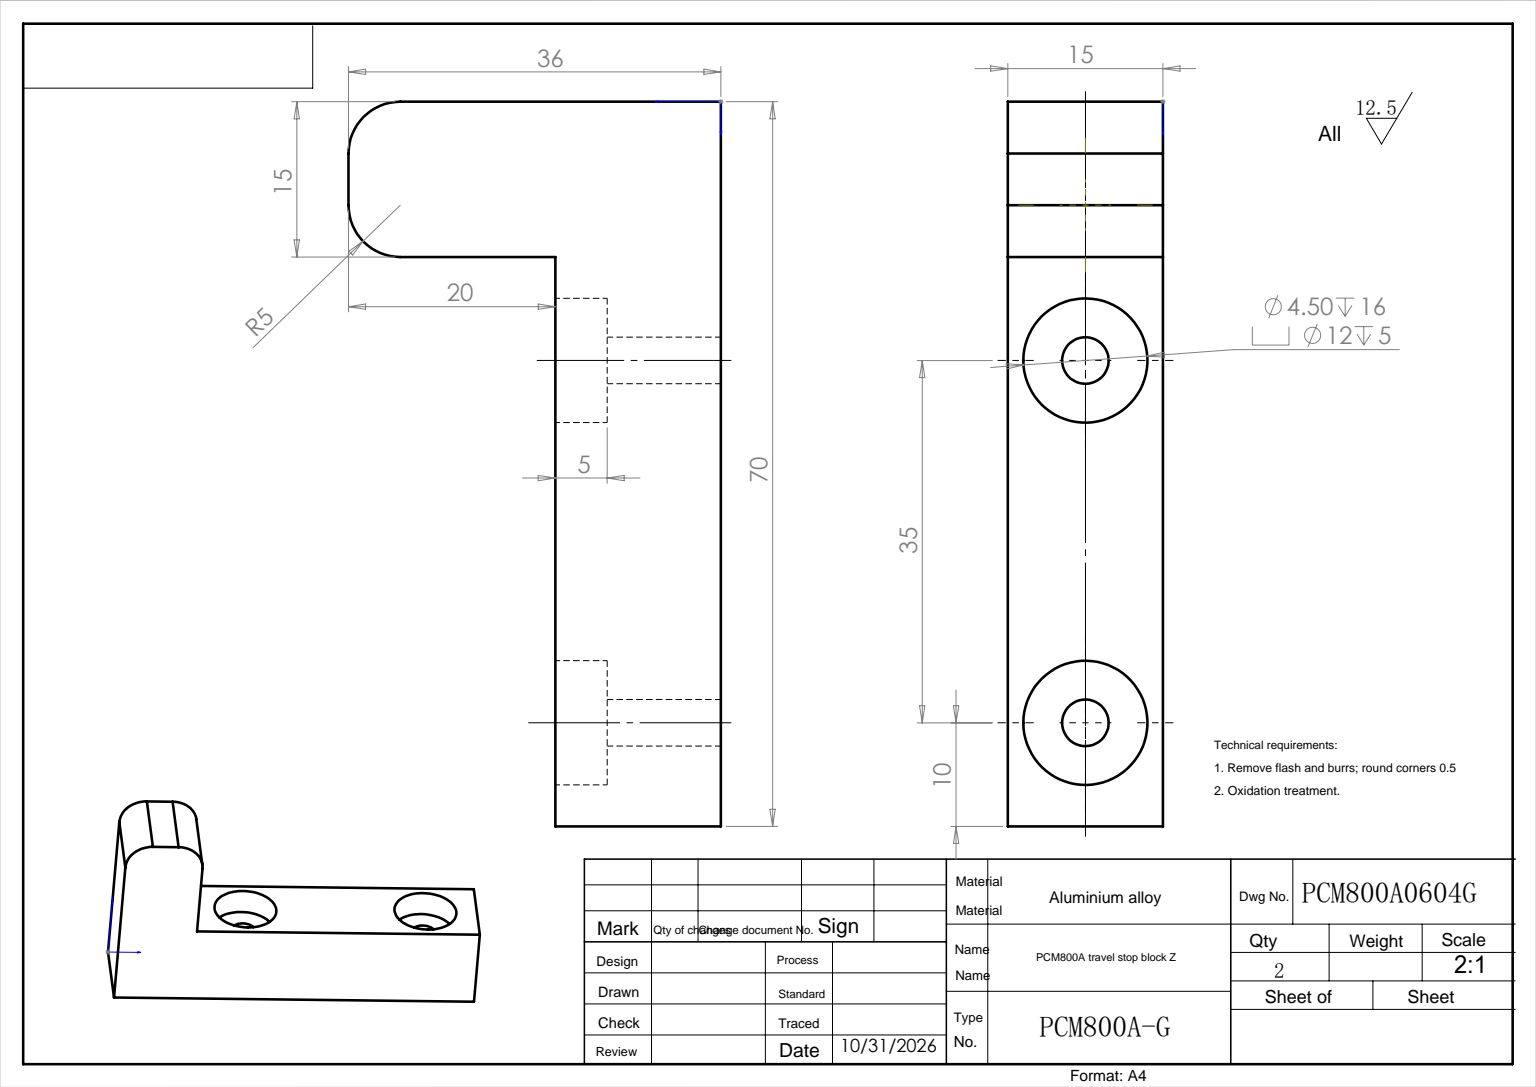
SolidWorks part; units mm, degrees
ref_plane "前视基准面" through (0, 0, 0) normal (0, 0, 1) x (1, 0, 0)
ref_plane "上视基准面" through (0, 0, 0) normal (0, 1, 0) x (1, 0, 0)
ref_plane "右视基准面" through (0, 0, 0) normal (1, 0, 0) x (0, 0, -1)
sketch "草图1" plane through (0, 0, 0) normal (0, 0, 1) x (1, 0, 0)
  line L0 (0, 0) -> (70, 0)
  line L1 (70, 0) -> (70, 16)
  line L2 (70, 16) -> (15, 16)
  line L3 (15, 16) -> (15, 36)
  line L4 (15, 36) -> (0, 36)
  line L5 (0, 36) -> (0, 16)
  line L7 (0, 16) -> (0, 0)
  dimension "D1" = 55
  dimension "D2" = 15
  dimension "D3" = 16
  dimension "D5" = 16
  dimension "D6" = 20
extrude "凸台-拉伸1" add sketch "草图1" along normal blind 15
fillet "圆角1" radius 5 2 edges at (0, 36, 7.5) (15, 36, 7.5)
hole_wizard "孔1" positions "草图5" profile "草图4" legacy
sketch "草图5" plane through (0, 16, 0) normal (0, 1, 0) x (-1, 0, 0)
  line L0 (-70, 7.5) -> (13.584, 7.5) construction
  line L1 (-70, 15) -> (-70, 0) construction
  point P0 (-25, 7.5)
  point P1 (-60, 7.5)
  dimension "D1" = 10
  dimension "D2" = 35
sketch "草图4" plane through (25, 16, 7.5) normal (1, 0, 0) x (0, 0, 1)
  line L0 (0, 0) -> (0, 100)
  line L1 (0, 100) -> (2.25, 100)
  line L2 (2.25, 100) -> (2.25, 5)
  line L3 (2.25, 5) -> (6, 5)
  line L4 (6, 5) -> (6, 0)
  line L5 (6, 0) -> (0, 0)
  line L6 (0, 110) -> (0, -10) construction
  dimension "直径" = 4.5
  dimension "深度" = 100
  dimension "柱坑直径" = 12
  dimension "柱坑深度" = 5
